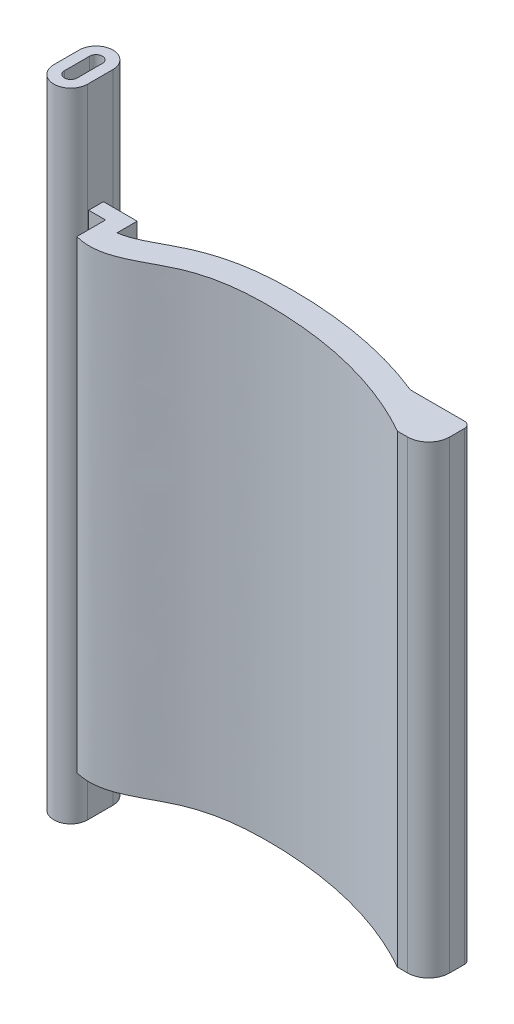
SolidWorks part; units mm, degrees
ref_plane "Front Plane" through (0, 0, 0) normal (0, 0, 1) x (1, 0, 0)
ref_plane "Top Plane" through (0, 0, 0) normal (0, 1, 0) x (1, 0, 0)
ref_plane "Right Plane" through (0, 0, 0) normal (1, 0, 0) x (0, 0, -1)
other "Configuration Table"
sketch "Sketch1" plane through (0, 0, 0) normal (0, 1, 0) x (1, 0, 0)
  line L0 (0, 11.4968) -> (0, -0.5032) construction
  line L1 (3, 11.4968) -> (3, -0.5032)
  line L2 (-3, 11.4968) -> (-3, -0.5032)
  arc A0 (3, 11.4968) -> (-3, 11.4968) centre (0, 11.4968) ccw
  arc A1 (-3, -0.5032) -> (3, -0.5032) centre (0, -0.5032) ccw
  point P3 (0, 5.4968)
  dimension "D2" = 3
  dimension "D1" = 12
extrude "Extrude-Thin1" add sketch "Sketch1" against normal blind 300 and the other way blind 2 thin thin type one direction wall 5
sketch "Sketch3" plane through (0, 0, 0) normal (0, 1, 0) x (1, 0, 0)
  line L0 (8, 0) -> (16, 0)
  line L1 (8, -0.5032) -> (8, 11.4968) construction
  line L2 (16, 0) -> (16, -13.6213)
  line L3 (171.8492, -17.5115) -> (176.6132, -17.5115)
  line L4 (8, 7) -> (24, 7)
  line L5 (24, 7) -> (24, -2.5146)
  line L6 (158, 2.4885) -> (183.6132, 2.4885)
  line L7 (8, 0) -> (8, 7)
  line L8 (8, 3.5) -> (238, 3.5) construction
  line L9 (186.6132, -7.5115) -> (186.6132, -0.5115)
  arc A0 (176.6132, -17.5115) -> (186.6132, -7.5115) centre (176.6132, -7.5115) ccw
  arc A1 (186.6132, -0.5115) -> (183.6132, 2.4885) centre (183.6132, -0.5115) ccw
  spline S0 degree 3 poles (16, -13.6213) (30.4999, -17.6446) (51.9364, 1.3106) (107.3097, 6.1573) (147.0968, -3.4849) (171.8492, -17.5115) knots 0 0 0 0 0.250268 0.483181 1 1 1 1
  spline S1 degree 1 poles (19.2084, -2.0581) (177.7655, -7.0713) knots 0 0 1 1 construction
  spline S2 degree 3 poles (19.2084, -2.0581) (19.4546, -2.1264) (19.9607, -2.2528) (20.9031, -2.4354) (22.0213, -2.5618) (23.0023, -2.5729) (23.7737, -2.5351) (24.235, -2.496) (25.5095, -2.3417) (27.6007, -1.8832) (31.0102, -0.6263) (34.88, 1.2138) (39.1863, 3.5006) (43.1601, 5.6175) (46.6014, 7.3146) (49.3486, 8.563) (52.1931, 9.7114) (55.9827, 11.0627) (60.7578, 12.4562) (66.4946, 13.7028) (74.1215, 14.8747) (81.6653, 15.4206) (89.0558, 15.5401) (96.3117, 15.4426) (105.3616, 14.9559) (119.7288, 13.3634) (136.5666, 9.9924) (151.2373, 5.2409) (161.3626, 1.1317) (168.8392, -2.2575) (174.5598, -5.2547) (177.7655, -7.0713) knots 0 0 0 0 0.007812 0.015625 0.03125 0.046537 0.050443 0.058255 0.0625 0.09375 0.125 0.15625 0.1875 0.21875 0.234375 0.25 0.265625 0.28125 0.3125 0.34375 0.375 0.4375 0.46875 0.5 0.5625 0.625 0.75 0.859647 0.890897 0.9375 1 1 1 1 only from (24, -2.5146) to (158, 2.4885)
  dimension "D5" = 12
  dimension "D7" = 150
  dimension "D8" = 10
  dimension "D9" = 3
  dimension "D1" = 8
  dimension "D2" = 16
  dimension "D3" = 7
  dimension "D4" = 230
  dimension "D6" = 20
extrude "Boss-Extrude1" add sketch "Sketch3" against normal blind 220 from offset 50
